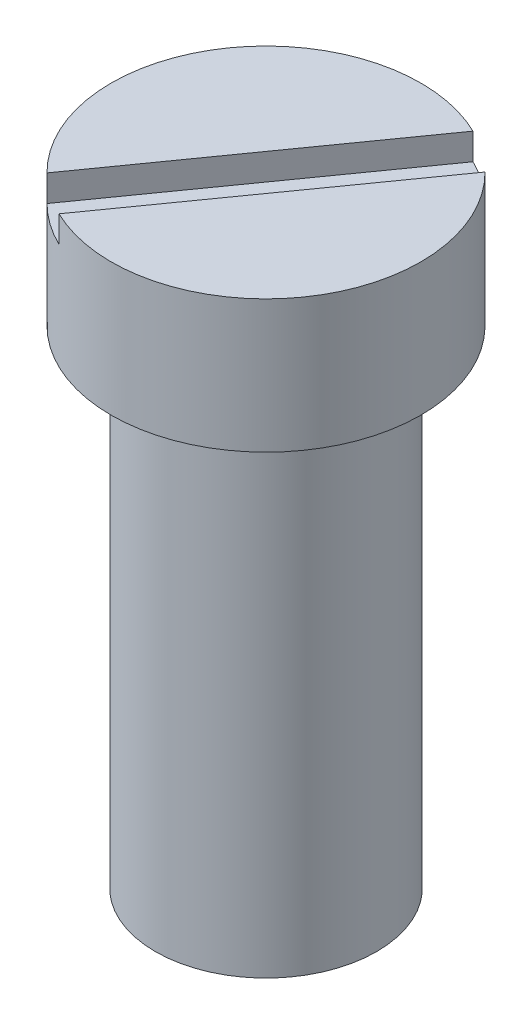
SolidWorks part; units mm, degrees
ref_plane "Front Plane" through (0, 0, 0) normal (0, 0, 1) x (1, 0, 0)
ref_plane "Top Plane" through (0, 0, 0) normal (0, 1, 0) x (1, 0, 0)
ref_plane "Right Plane" through (0, 0, 0) normal (1, 0, 0) x (0, 0, -1)
sketch "Sketch1" plane through (0, 0, 0) normal (0, 1, 0) x (1, 0, 0)
  circle A0 centre (0, 0) radius 1.25
  dimension "D1" = 2.5
extrude "Boss-Extrude1" add sketch "Sketch1" along normal blind 5.5
sketch "Sketch2" plane through (0, 5.5, 0) normal (0, 1, 0) x (1, 0, 0)
  circle A0 centre (0, 0) radius 1.75
  circle A1 centre (0, 0) radius 1.25 construction
  dimension "D1" = 0.5
extrude "Boss-Extrude2" add sketch "Sketch2" along normal blind 1.5
sketch "Sketch3" plane through (0, 7, 0) normal (0, 1, 0) x (1, 0, 0)
  line L0 (-1.6118, -1.7754) -> (1.1435, 2.1077)
  line L1 (-1.6118, -1.7754) -> (-1.1435, -2.1077)
  line L2 (1.1435, 2.1077) -> (1.6118, 1.7754)
  line L3 (-1.1435, -2.1077) -> (1.6118, 1.7754)
  line L4 (-1.6118, -1.7754) -> (1.6118, 1.7754) construction
  line L5 (1.1435, 2.1077) -> (-1.1435, -2.1077) construction
  point P1 (0, 0)
extrude "Cut-Extrude1" cut sketch "Sketch3" against normal blind 0.3
